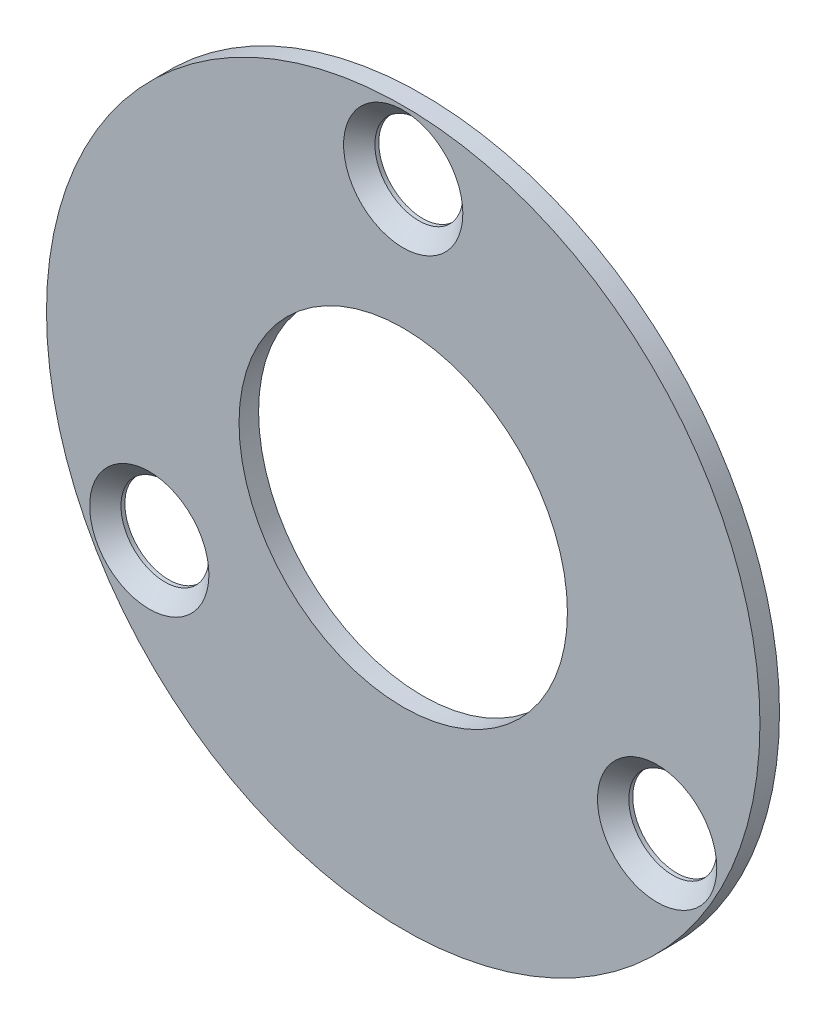
SolidWorks part; units mm, degrees
material "铁Q235"
ref_plane "前视基准面" through (0, 0, 0) normal (0, 0, 1) x (1, 0, 0)
ref_plane "上视基准面" through (0, 0, 0) normal (0, 1, 0) x (1, 0, 0)
ref_plane "右视基准面" through (0, 0, 0) normal (1, 0, 0) x (0, 0, -1)
sketch "草图1" plane through (0, 0, 0) normal (0, 0, 1) x (1, 0, 0)
  circle A0 centre (0, 0) radius 18.25
  circle A1 centre (0, 0) radius 8.4
  circle A2 centre (0, 0) radius 15 construction
  circle A3 centre (0, 15) radius 2.25
  circle A4 centre (12.9904, -7.5) radius 2.25
  circle A5 centre (-12.9904, -7.5) radius 2.25
  point P14 (0, 0)
  dimension "D1" = 36.5
  dimension "D2" = 3
  dimension "D3" = 30
extrude "凸台-拉伸1" add sketch "草图1" along normal blind 1
chamfer "倒角1" distance 0.8 angle 45 3 edges at (15.2404, -7.5, 1) (-10.7404, -7.5, 1) (2.25, 15, 1)
